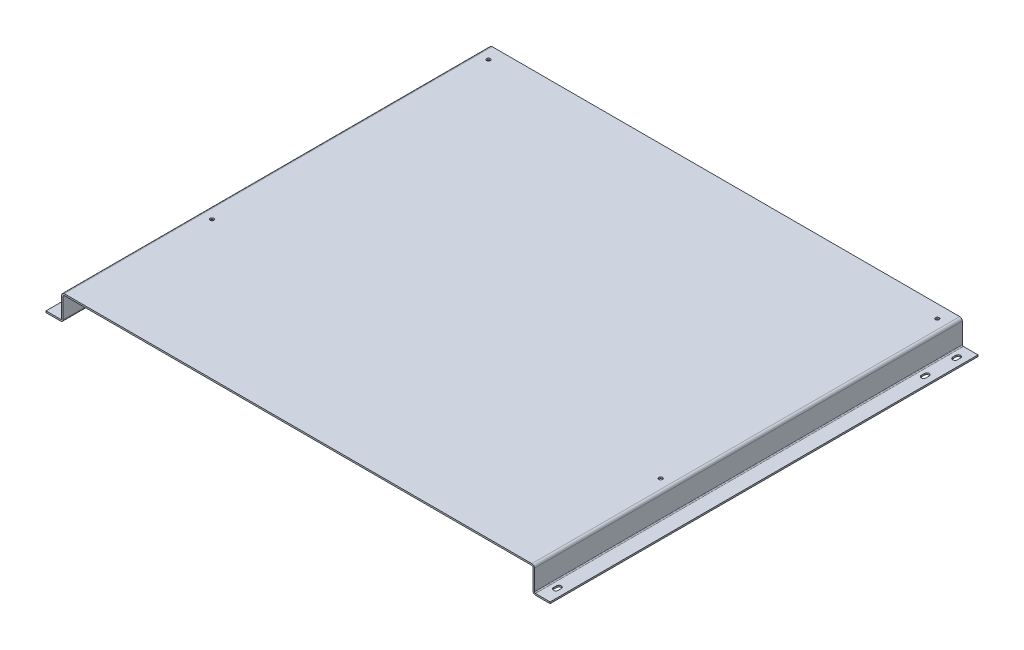
from build123d import *

# Parameters (mm, degrees)
EXTRUDE_1_DEPTH     = 820
SKETCH_2_R          = 3.5
CUT_EXTRUDE_1_DEPTH = 820
CUT_EXTRUDE_2_DEPTH = 10


with BuildPart() as part:
    # 草图1 → 凸台-拉伸1 (new body)
    with BuildSketch(Plane.XY):
        with BuildLine():
            Line((0, 0), (28, 0))
            ThreePointArc((28, 0), (29.414213562, 0.585786438), (30, 2))
            Line((30, 2), (30, 41))
            ThreePointArc((30, 41), (31.464466094, 44.535533906), (35, 46))
            Line((35, 46), (931, 46))
            ThreePointArc((931, 46), (934.535533906, 44.535533906), (936, 41))
            Line((936, 41), (936, 2))
            ThreePointArc((936, 2), (936.585786438, 0.585786438), (938, 0))
            Line((938, 0), (966, 0))
            Line((966, 0), (966, -3))
            Line((966, -3), (938, -3))
            ThreePointArc((938, -3), (934.464466094, -1.535533906), (933, 2))
            Line((933, 2), (933, 41))
            ThreePointArc((933, 41), (932.414213562, 42.414213562), (931, 43))
            Line((931, 43), (35, 43))
            ThreePointArc((35, 43), (33.585786438, 42.414213562), (33, 41))
            Line((33, 41), (33, 2))
            ThreePointArc((33, 2), (31.535533906, -1.535533906), (28, -3))
            Line((28, -3), (0, -3))
            Line((0, -3), (0, 0))
        make_face()
    extrude(amount=EXTRUDE_1_DEPTH)

    # 草图2 → 切除-拉伸1 (cut)
    with BuildSketch(Plane(origin=(0, 46, 0), x_dir=(1, 0, 0), z_dir=(0, 1, 0))):
        with Locations(Location((53, -555, 0), (0, 0, 270))):
            Circle(SKETCH_2_R)
        with Locations(Location((53, -25, 0), (0, 0, 270))):
            Circle(SKETCH_2_R)
        with Locations(Location((913, -25, 0), (0, 0, 270))):
            Circle(SKETCH_2_R)
        with Locations(Location((913, -555, 0), (0, 0, 270))):
            Circle(SKETCH_2_R)
    extrude(amount=-CUT_EXTRUDE_1_DEPTH, mode=Mode.SUBTRACT)

    # 草图3 → 切除-拉伸2 (cut)
    with BuildSketch(Plane(origin=(0, 0, 0), x_dir=(1, 0, 0), z_dir=(0, 1, 0))):
        with BuildLine():
            Line((954.5, -82), (954.5, -88))
            ThreePointArc((954.5, -88), (950, -92.5), (945.5, -88))
            Line((945.5, -88), (945.5, -82))
            ThreePointArc((945.5, -82), (950, -77.5), (954.5, -82))
        make_face()
        with BuildLine():
            Line((954.5, -22), (954.5, -28))
            ThreePointArc((954.5, -28), (950, -32.5), (945.5, -28))
            Line((945.5, -28), (945.5, -22))
            ThreePointArc((945.5, -22), (950, -17.5), (954.5, -22))
        make_face()
        with BuildLine():
            Line((11.5, -82), (11.5, -88))
            ThreePointArc((11.5, -88), (16, -92.5), (20.5, -88))
            Line((20.5, -88), (20.5, -82))
            ThreePointArc((20.5, -82), (16, -77.5), (11.5, -82))
        make_face()
        with BuildLine():
            Line((11.5, -22), (11.5, -28))
            ThreePointArc((11.5, -28), (16, -32.5), (20.5, -28))
            Line((20.5, -28), (20.5, -22))
            ThreePointArc((20.5, -22), (16, -17.5), (11.5, -22))
        make_face()
        with BuildLine():
            Line((954.5, -787), (954.5, -793))
            ThreePointArc((954.5, -793), (950, -797.5), (945.5, -793))
            Line((945.5, -793), (945.5, -787))
            ThreePointArc((945.5, -787), (950, -782.5), (954.5, -787))
        make_face()
        with BuildLine():
            Line((11.5, -787), (11.5, -793))
            ThreePointArc((11.5, -793), (16, -797.5), (20.5, -793))
            Line((20.5, -793), (20.5, -787))
            ThreePointArc((20.5, -787), (16, -782.5), (11.5, -787))
        make_face()
    extrude(amount=-CUT_EXTRUDE_2_DEPTH, mode=Mode.SUBTRACT)


solid = part.part
